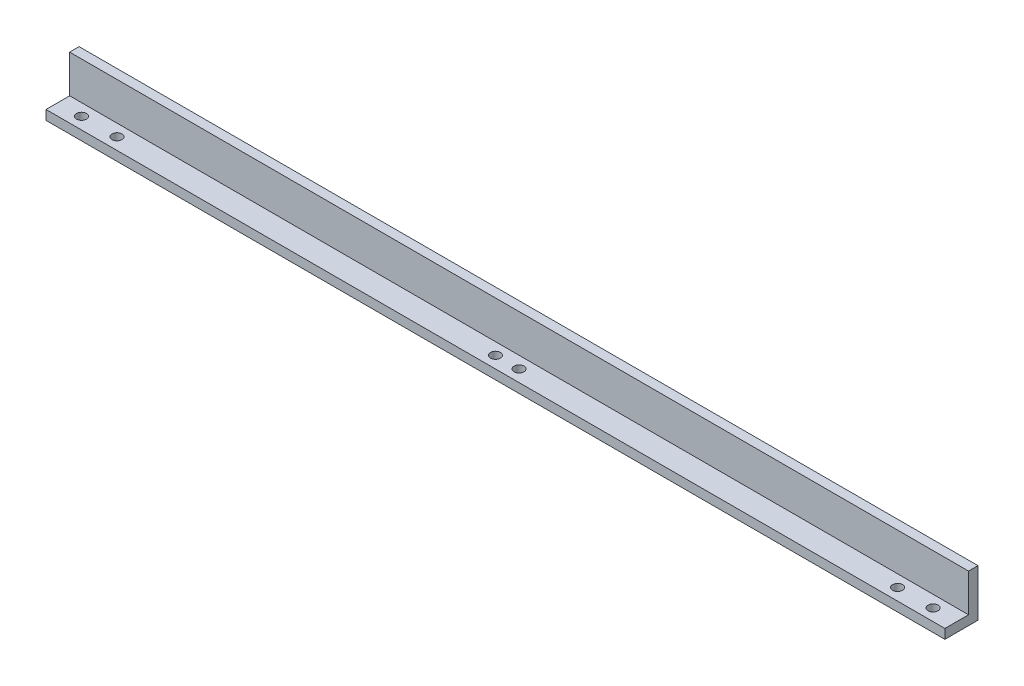
from build123d import *

# Parameters (mm, degrees)
SKETCH1_W           = 380
SKETCH1_H           = 10
SKETCH1_R           = 2.1
BOSS_EXTRUDE1_DEPTH = 4
SKETCH2_W           = 380
SKETCH2_H           = 20
BOSS_EXTRUDE2_DEPTH = 4


with BuildPart() as part:
    # Sketch1 → Boss-Extrude1 (new body)
    with BuildSketch(Plane(origin=(0, 0, 0), x_dir=(1, 0, 0), z_dir=(0, 1, 0))):
        Rectangle(SKETCH1_W, SKETCH1_H)
        with Locations(Location((-180, 0, 0), (0, 0, 270))):
            Circle(SKETCH1_R, mode=Mode.SUBTRACT)
        with Locations(Location((-165, 0, 0), (0, 0, 270))):
            Circle(SKETCH1_R, mode=Mode.SUBTRACT)
        with Locations(Location((165, 0, 0), (0, 0, 90))):
            Circle(SKETCH1_R, mode=Mode.SUBTRACT)
        with Locations(Location((180, 0, 0), (0, 0, 90))):
            Circle(SKETCH1_R, mode=Mode.SUBTRACT)
        with Locations(Location((5, 0, 0), (0, 0, 270))):
            Circle(SKETCH1_R, mode=Mode.SUBTRACT)
        with Locations(Location((-5, 0, 0), (0, 0, 270))):
            Circle(SKETCH1_R, mode=Mode.SUBTRACT)
    extrude(amount=BOSS_EXTRUDE1_DEPTH)

    # Sketch2 → Boss-Extrude2 (add)
    with BuildSketch(Plane(origin=(0, 0, -5), x_dir=(-1, 0, 0), z_dir=(0, 0, -1))):
        with Locations((0, 10)):
            Rectangle(SKETCH2_W, SKETCH2_H)
    extrude(amount=BOSS_EXTRUDE2_DEPTH)


solid = part.part
